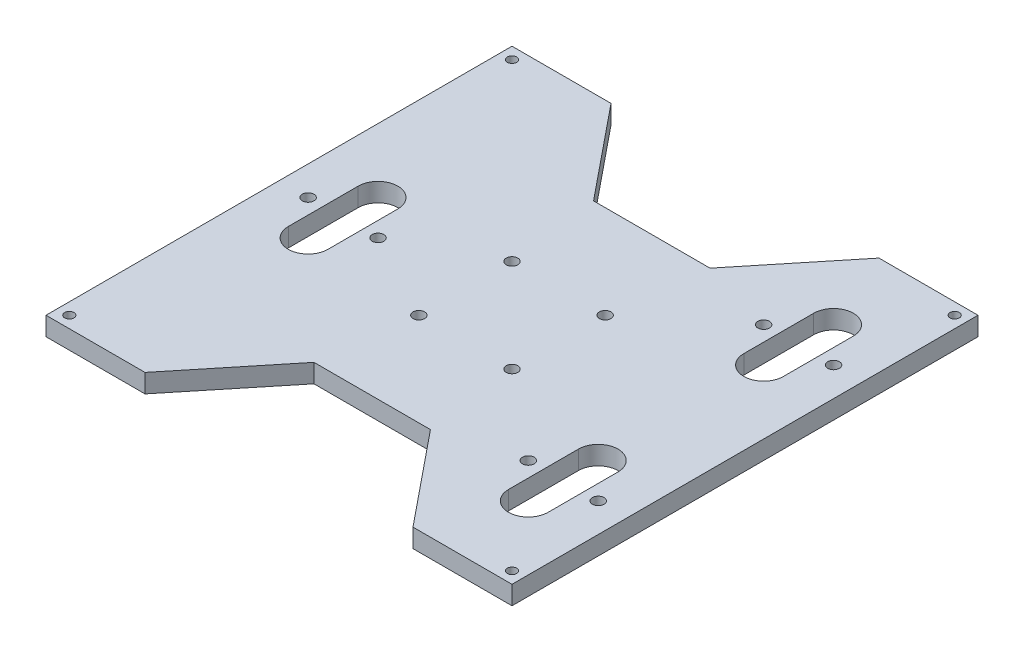
SolidWorks part; units mm, degrees
material "Beech"
ref_plane "Front Plane" through (0, 0, 0) normal (0, 0, 1) x (1, 0, 0)
ref_plane "Top Plane" through (0, 0, 0) normal (0, 1, 0) x (1, 0, 0)
ref_plane "Right Plane" through (0, 0, 0) normal (1, 0, 0) x (0, 0, -1)
sketch "Sketch1" plane through (0, 0, 0) normal (0, 1, 0) x (1, 0, 0)
  line L0 (0, 100) -> (200, 100) construction
  line L1 (0, 0) -> (200, 0)
  line L2 (0, 0) -> (0, 200)
  line L3 (0, 200) -> (200, 200)
  line L4 (200, 0) -> (200, 200)
  line L5 (100, 200) -> (100, 0) construction
  circle A0 centre (195, 195) radius 2
  circle A1 centre (5, 195) radius 2
  circle A2 centre (5, 5) radius 2
  circle A3 centre (195, 5) radius 2
  dimension "D3" = 190
  dimension "D4" = 190
  dimension "D5" = 4
  dimension "D1" = 200
  dimension "D2" = 200
extrude "Boss-Extrude1" add sketch "Sketch1" along normal blind 8
sketch "Sketch2" plane through (0, 0, 0) normal (0, -1, 0) x (1, 0, 0)
  line L0 (200, 0) -> (200, -200) construction
  line L1 (0, 0) -> (200, 0) construction
  line L2 (0, -100) -> (53.9274, -100) construction
  line L3 (0, -200) -> (0, 0) construction
  line L4 (0, -100) -> (200, -100) construction
  line L5 (100, 0) -> (100, -200) construction
  line L6 (200, -200) -> (0, -200) construction
  circle A0 centre (187.5, -49.5) radius 2.5
  circle A1 centre (157.5, -49.5) radius 2.5
  circle A2 centre (80, -120) radius 2.5
  circle A3 centre (80, -80) radius 2.5
  circle A4 centre (120, -80) radius 2.5
  circle A5 centre (120, -120) radius 2.5
  circle A6 centre (42.5, -100) radius 2.5
  circle A7 centre (12.5, -100) radius 2.5
  circle A10 centre (157.5, -150.5) radius 2.5
  circle A11 centre (187.5, -150.5) radius 2.5
  dimension "D1" = 5
  dimension "D2" = 30
  dimension "D3" = 30
  dimension "D8" = 40
  dimension "D9" = 40
  dimension "D4" = 12.5
  dimension "D5" = 157.5
  dimension "D6" = 49.5
  dimension "D7" = 150.5
extrude "Cut-Extrude1" cut sketch "Sketch2" against normal through all
sketch "Sketch3" plane through (0, 8, 0) normal (0, 1, 0) x (1, 0, 0)
  line L0 (100, 0) -> (100, 200) construction
  line L1 (0, 0) -> (200, 0) construction
  line L2 (200, 200) -> (0, 200) construction
  line L3 (0, 100) -> (200, 100) construction
  line L4 (0, 200) -> (0, 0) construction
  line L5 (200, 0) -> (200, 200) construction
  line L6 (42.5, 200) -> (75, 160)
  line L7 (157.5, 200) -> (125, 160)
  line L8 (75, 160) -> (125, 160)
  line L9 (42.5, 200) -> (157.5, 200)
  line L10 (187.5, 49.5) -> (157.5, 49.5) construction
  line L11 (172.5, 49.5) -> (172.5, 76.3951) construction
  line L18 (42.5, 0) -> (157.5, 0)
  line L19 (75, 40) -> (125, 40)
  line L20 (157.5, 0) -> (125, 40)
  line L21 (42.5, 0) -> (75, 40)
  line L25 (19, 85) -> (19, 115)
  line L27 (36, 85) -> (36, 115)
  line L33 (181, 34.5) -> (181, 64.5)
  line L34 (164, 34.5) -> (164, 64.5)
  line L37 (181, 165.5) -> (181, 135.5)
  line L39 (164, 165.5) -> (164, 135.5)
  line L40 (172.5, 165.5) -> (172.5, 135.5) construction
  arc A0 (164, 135.5) -> (181, 135.5) centre (172.5, 135.5) ccw
  arc A1 (181, 165.5) -> (164, 165.5) centre (172.5, 165.5) ccw
  arc A2 (181, 64.5) -> (164, 64.5) centre (172.5, 64.5) ccw
  arc A3 (164, 34.5) -> (181, 34.5) centre (172.5, 34.5) ccw
  arc A4 (19, 85) -> (36, 85) centre (27.5, 85) ccw
  arc A5 (36, 115) -> (19, 115) centre (27.5, 115) ccw
  point P16 (100, 160)
  point P27 (100, 40)
  dimension "D1" = 50
  dimension "D2" = 40
  dimension "D3" = 115
  dimension "D4" = 17
  dimension "D5" = 30
  dimension "D7" = 17
  dimension "D8" = 30
  dimension "D9" = 17
  dimension "D10" = 30
extrude "Cut-Extrude2" cut sketch "Sketch3" against normal through all
